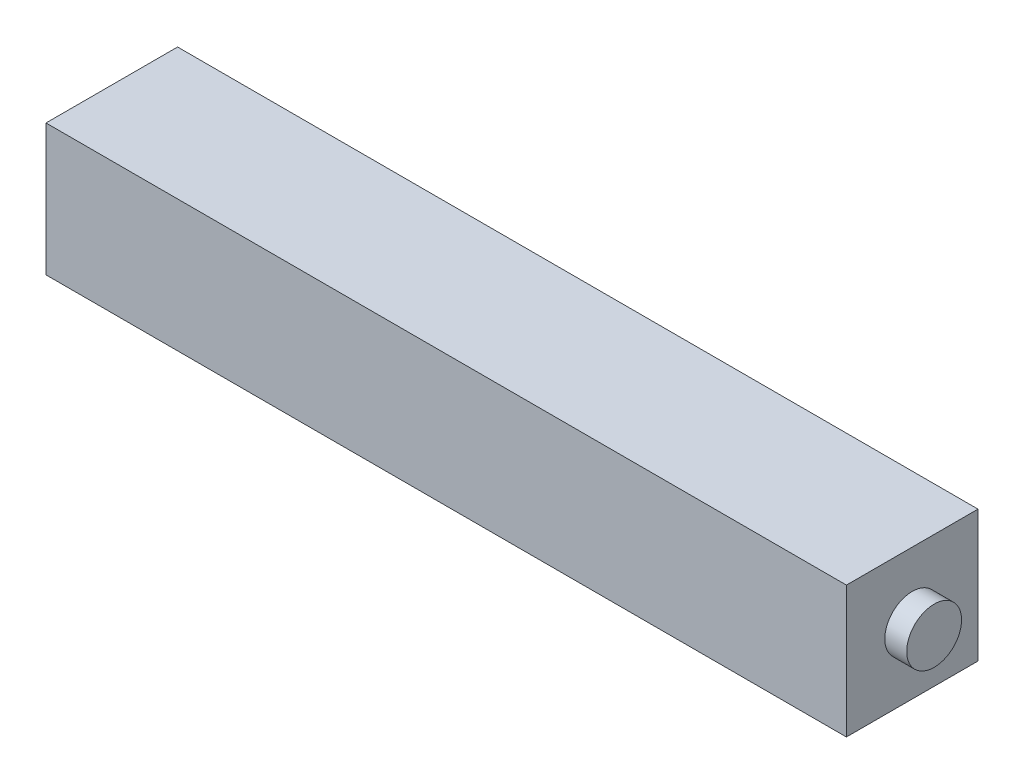
SolidWorks part; units mm, degrees
ref_plane "Front Plane" through (0, 0, 0) normal (0, 0, 1) x (1, 0, 0)
ref_plane "Top Plane" through (0, 0, 0) normal (0, 1, 0) x (1, 0, 0)
ref_plane "Right Plane" through (0, 0, 0) normal (1, 0, 0) x (0, 0, -1)
sketch "Sketch1" plane through (0, 0, 0) normal (0, 0, 1) x (1, 0, 0)
  line L1 (-37.5, 6) -> (37.5, 6)
  line L2 (-37.5, 6) -> (-37.5, -6)
  line L3 (-37.5, -6) -> (37.5, -6)
  line L4 (37.5, 6) -> (37.5, -6)
  line L5 (-37.5, 6) -> (37.5, -6) construction
  line L6 (-37.5, -6) -> (37.5, 6) construction
  point P0 (0, 0)
  dimension "D1" = 12
  dimension "D2" = 75
extrude "Boss-Extrude1" add sketch "Sketch1" along normal blind 12
sketch "Sketch2" plane through (37.5, 0, 0) normal (1, 0, 0) x (0, 0, -1)
  line L0 (-12, 0) -> (0, 0) construction
  line L1 (-12, -6) -> (-12, 6) construction
  circle A0 centre (-6, 0) radius 2.5
  dimension "D1" = 5
extrude "Cut-Extrude1" cut sketch "Sketch2" against normal blind 2 flip side to cut
